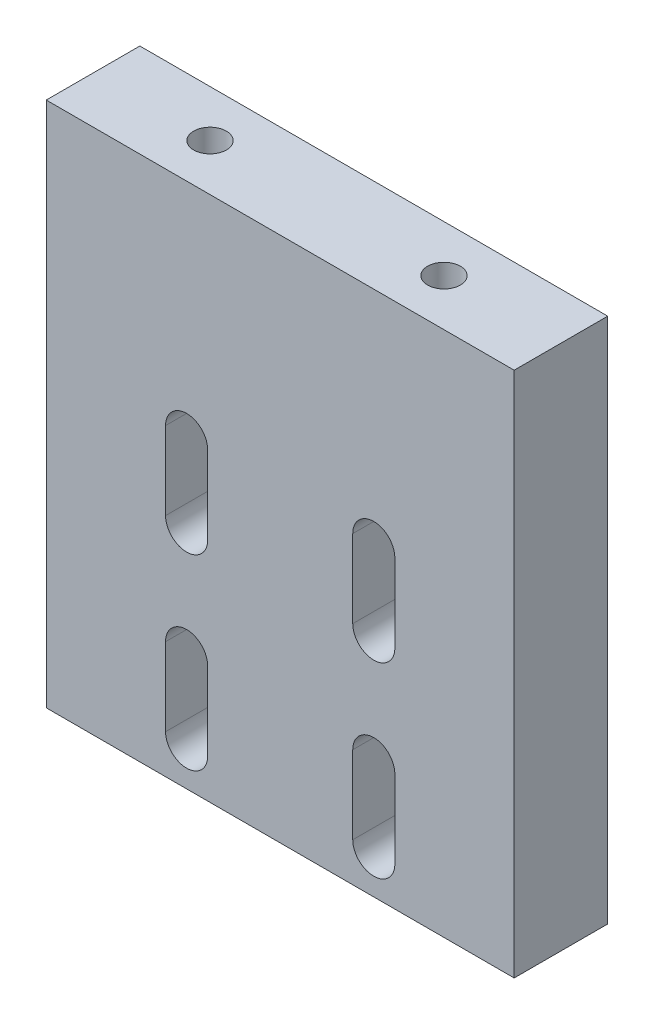
SolidWorks part; units mm, degrees
material "6061 合金"
ref_plane "前基準面" through (0, 0, 0) normal (0, 0, 1) x (1, 0, 0)
ref_plane "上基準面" through (0, 0, 0) normal (0, 1, 0) x (1, 0, 0)
ref_plane "右基準面" through (0, 0, 0) normal (1, 0, 0) x (0, 0, -1)
sketch "草图1" plane through (0, 0, 0) normal (0, 0, 1) x (1, 0, 0)
  line L1 (-30, 33.75) -> (30, 33.75)
  line L2 (-30, 33.75) -> (-30, -33.75)
  line L3 (-30, -33.75) -> (30, -33.75)
  line L4 (30, 33.75) -> (30, -33.75)
  line L5 (-30, 33.75) -> (30, -33.75) construction
  line L6 (-30, -33.75) -> (30, 33.75) construction
  point P0 (0, 0)
  dimension "D1" = 60
  dimension "D2" = 67.5
extrude "凸台-拉伸1" add sketch "草图1" along normal mid plane 12
sketch "草图2" plane through (0, 0, -6) normal (0, 0, -1) x (-1, 0, 0)
  line L0 (12, -28.75) -> (12, -18.75) construction
  line L1 (9.3, -28.75) -> (9.3, -18.75)
  line L2 (14.7, -28.75) -> (14.7, -18.75)
  line L3 (-12, -28.75) -> (-12, -18.75) construction
  line L4 (-14.7, -28.75) -> (-14.7, -18.75)
  line L5 (-9.3, -28.75) -> (-9.3, -18.75)
  line L6 (12, 5.25) -> (12, -4.75) construction
  line L7 (14.7, 5.25) -> (14.7, -4.75)
  line L8 (9.3, 5.25) -> (9.3, -4.75)
  line L9 (-12, 5.25) -> (-12, -4.75) construction
  line L10 (-9.3, 5.25) -> (-9.3, -4.75)
  line L11 (-14.7, 5.25) -> (-14.7, -4.75)
  arc A0 (9.3, -28.75) -> (14.7, -28.75) centre (12, -28.75) ccw
  arc A1 (14.7, -18.75) -> (9.3, -18.75) centre (12, -18.75) ccw
  arc A2 (-14.7, -28.75) -> (-9.3, -28.75) centre (-12, -28.75) ccw
  arc A3 (-9.3, -18.75) -> (-14.7, -18.75) centre (-12, -18.75) ccw
  arc A4 (14.7, 5.25) -> (9.3, 5.25) centre (12, 5.25) ccw
  arc A5 (9.3, -4.75) -> (14.7, -4.75) centre (12, -4.75) ccw
  arc A6 (-9.3, 5.25) -> (-14.7, 5.25) centre (-12, 5.25) ccw
  arc A7 (-14.7, -4.75) -> (-9.3, -4.75) centre (-12, -4.75) ccw
  point P2 (12, -23.75)
  point P10 (-12, -23.75)
  point P18 (12, 0.25)
  point P26 (-12, 0.25)
  dimension "D1" = 2.7
  dimension "D2" = 10
extrude "切除-拉伸1" cut sketch "草图2" against normal through all
hole_wizard "M5 螺纹孔1" positions "草图3" profile "草图4" tap size "M5" standard "ISO"
sketch "草图3" plane through (0, 33.75, 0) normal (0, 1, 0) x (1, 0, 0)
  line L0 (-15, 0) -> (0, 0) construction
  line L1 (0, 0) -> (15, 0) construction
  point P0 (-15, 0)
  point P2 (15, 0)
  dimension "D1" = 30
sketch "草图4" plane through (-15, 33.75, 0) normal (1, 0, 0) x (0, 0, 1)
  line L0 (0, 0) -> (0, 13.6618)
  line L1 (0, 13.6618) -> (2.1, 12.4)
  line L2 (2.1, 12.4) -> (2.1, 0)
  line L5 (2.1, 0) -> (0, 0)
  line L10 (0, 13.6618) -> (-2.1, 12.4) construction
  line L11 (0, -6.35) -> (0, 107.95) construction
  dimension "螺纹孔钻头直径" = 4.2
  dimension "螺纹孔钻头深度" = 12.4
  dimension "导头角度" = 118
cosmetic thread "孔螺蚊线1" parameters "D1"=10, "D2"=5
cosmetic thread "孔螺蚊线2" parameters "D1"=10, "D2"=5
